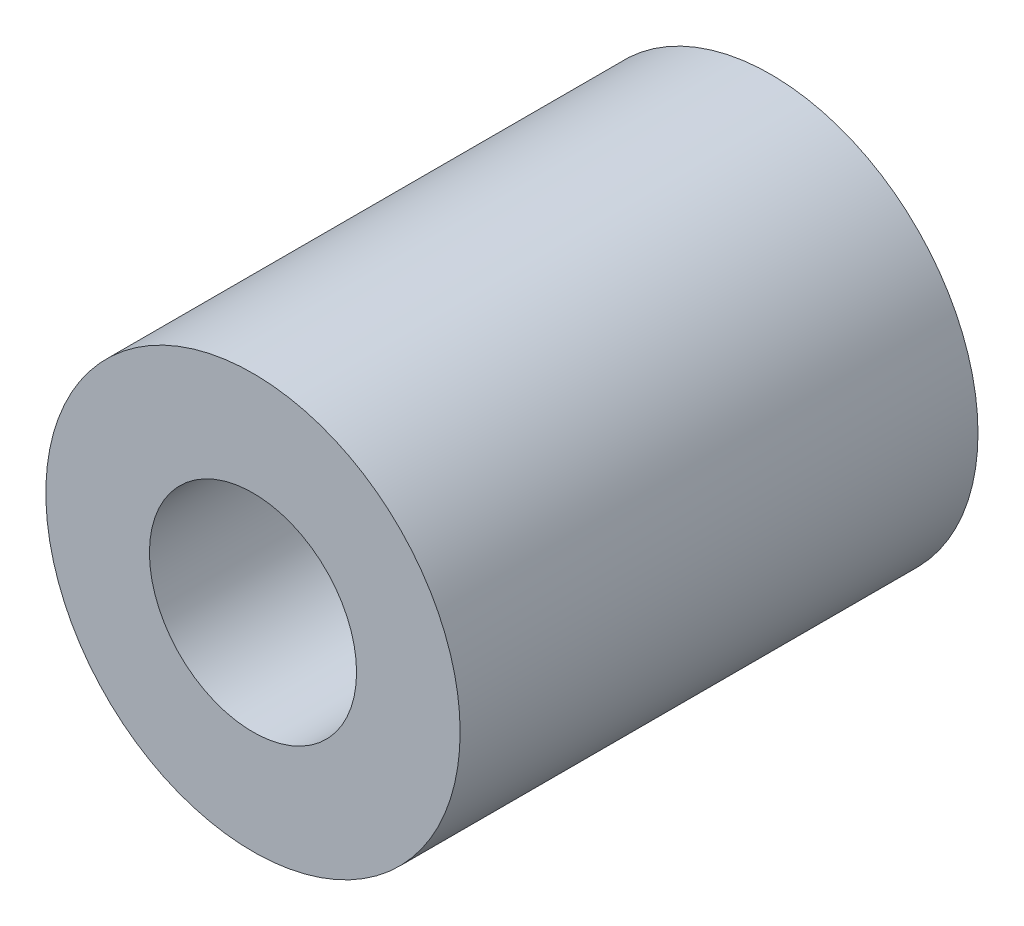
SolidWorks part; units mm, degrees
material "优力胶"
ref_plane "前视基准面" through (0, 0, 0) normal (0, 0, 1) x (1, 0, 0)
ref_plane "上视基准面" through (0, 0, 0) normal (0, 1, 0) x (1, 0, 0)
ref_plane "右视基准面" through (0, 0, 0) normal (1, 0, 0) x (0, 0, -1)
sketch "草图1" plane through (0, 0, 0) normal (0, 0, 1) x (1, 0, 0)
  circle A0 centre (0, 0) radius 6
  dimension "D1" = 12
extrude "凸台-拉伸1" add sketch "草图1" along normal blind 15
hole_wizard "打孔尺寸(%根据)内六角圆柱头螺钉的类型1" positions "草图2" profile "草图3" counterbore size "M4" standard "GB" end condition through all
sketch "草图2" plane through (0, 0, 15) normal (0, 0, 1) x (1, 0, 0)
  point P0 (0, 0)
sketch "草图3" plane through (0, 0, 15) normal (1, 0, 0) x (0, -1, 0)
  line L0 (0, 0) -> (0, 15)
  line L1 (0, 15) -> (1.65, 15)
  line L3 (1.65, 15) -> (1.65, 10)
  line L4 (1.65, 10) -> (3, 10)
  line L5 (3, 10) -> (3, 0)
  line L7 (3, 0) -> (0, 0)
  line L11 (0, -6.35) -> (0, 107.95) construction
  dimension "通孔孔直径" = 3.3
  dimension "通孔孔深度" = 15
  dimension "柱形沉头孔直径" = 6
  dimension "柱形沉头孔深度" = 10
